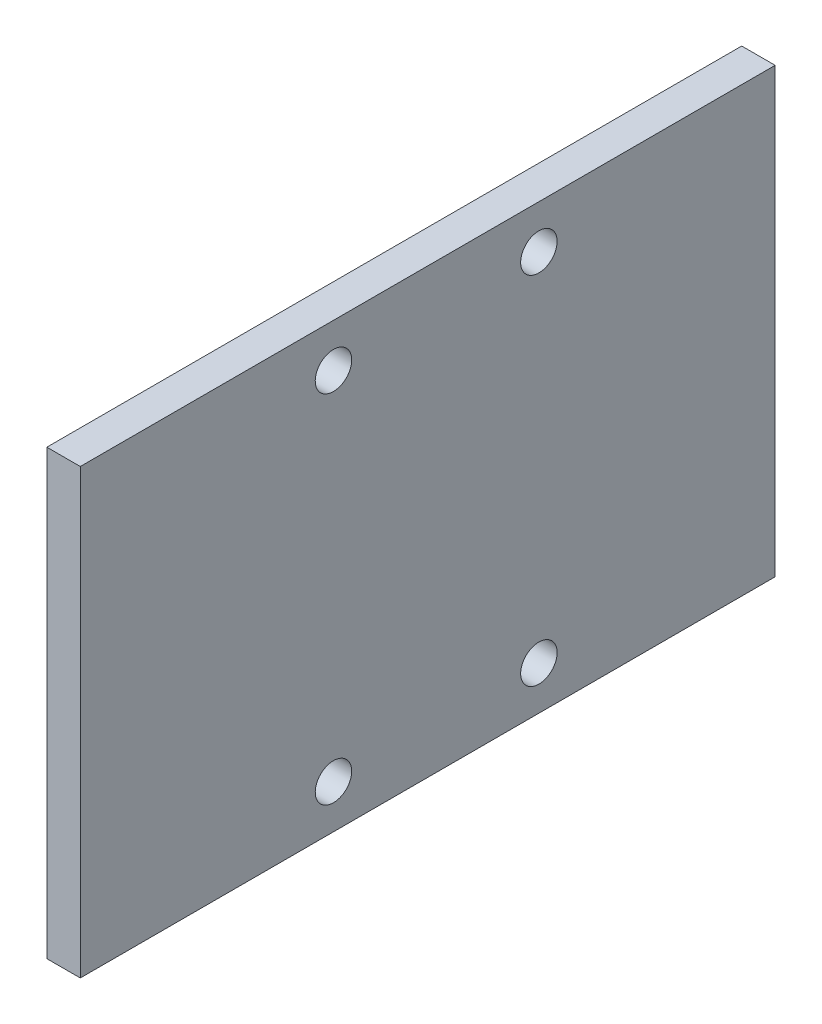
SolidWorks part; units mm, degrees
ref_plane "前视基准面" through (0, 0, 0) normal (0, 0, 1) x (1, 0, 0)
ref_plane "上视基准面" through (0, 0, 0) normal (0, 1, 0) x (1, 0, 0)
ref_plane "右视基准面" through (0, 0, 0) normal (1, 0, 0) x (0, 0, -1)
sketch "草图1" plane through (0, 0, 0) normal (0, 0, 1) x (1, 0, 0)
  line L1 (-2.3303, 8.4555) -> (1.5197, 8.4555)
  line L2 (-2.3303, 8.4555) -> (-2.3303, -42.5445)
  line L3 (-2.3303, -42.5445) -> (1.5197, -42.5445)
  line L4 (1.5197, 8.4555) -> (1.5197, -42.5445)
  dimension "D1" = 3.85
  dimension "D2" = 51
extrude "凸台-拉伸1" add sketch "草图1" along normal blind 80
extrude "切除-拉伸1" cut sketch "草图2" against normal up to surface (17.7 mm away)
sketch "草图2" plane through (5.3697, -1051.7947, 1009.1439) normal (1, 0, 0) x (0, -1, 0)
  line L0 (-1055.2503, 985.1439) -> (-1055.2503, 955.1439) construction
  line L3 (-1014.2503, 985.1439) -> (-1014.2503, 955.1439) construction
  line L6 (-1060.2503, 981.9423) -> (-1009.2503, 981.9423) construction
  line L9 (-1060.2503, 958.2923) -> (-1009.2503, 958.2923) construction
  circle A0 centre (-1055.2503, 981.9423) radius 2.1
  circle A1 centre (-1055.2503, 958.2923) radius 2.1
  circle A2 centre (-1014.2503, 958.2923) radius 2.1
  circle A3 centre (-1014.2503, 981.9423) radius 2.1
